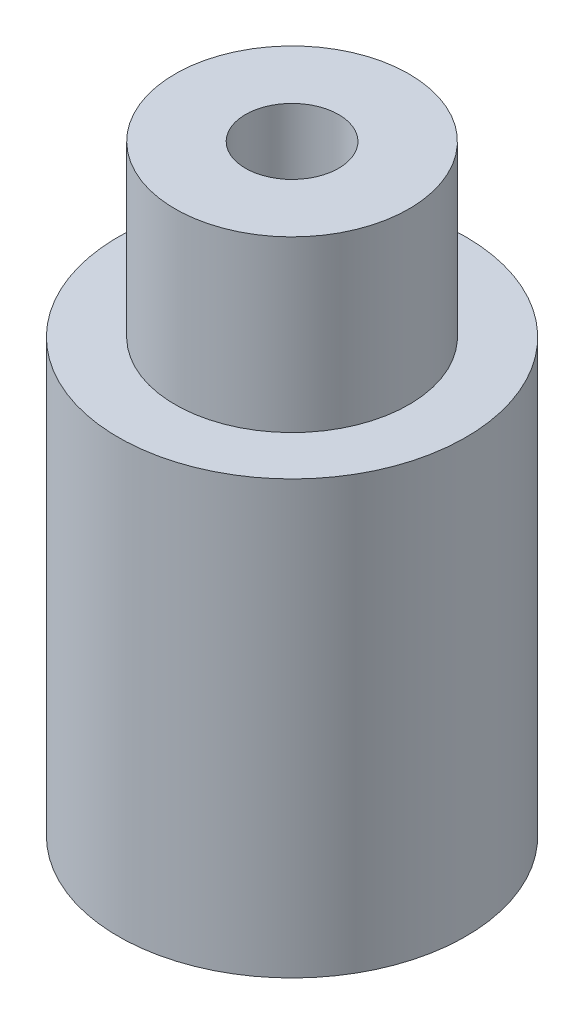
from build123d import *


with BuildPart() as part:
    # Sketch1 → Revolve1 (revolve)
    with BuildSketch(Plane.XY, mode=Mode.PRIVATE) as revolve1_sk:
        Polygon((-0.55, -1.5), (-2.05, -1.5), (-2.05, 3.6), (-1.38, 3.6), (-1.38, 5.6), (-0.55, 5.6), align=None)
    revolve(revolve1_sk.sketch.rotate(Axis((0, -0.731574036, 0), (0, 1, 0)), 270), axis=Axis((0, -0.731574036, 0), (0, 1, 0)))


solid = part.part
